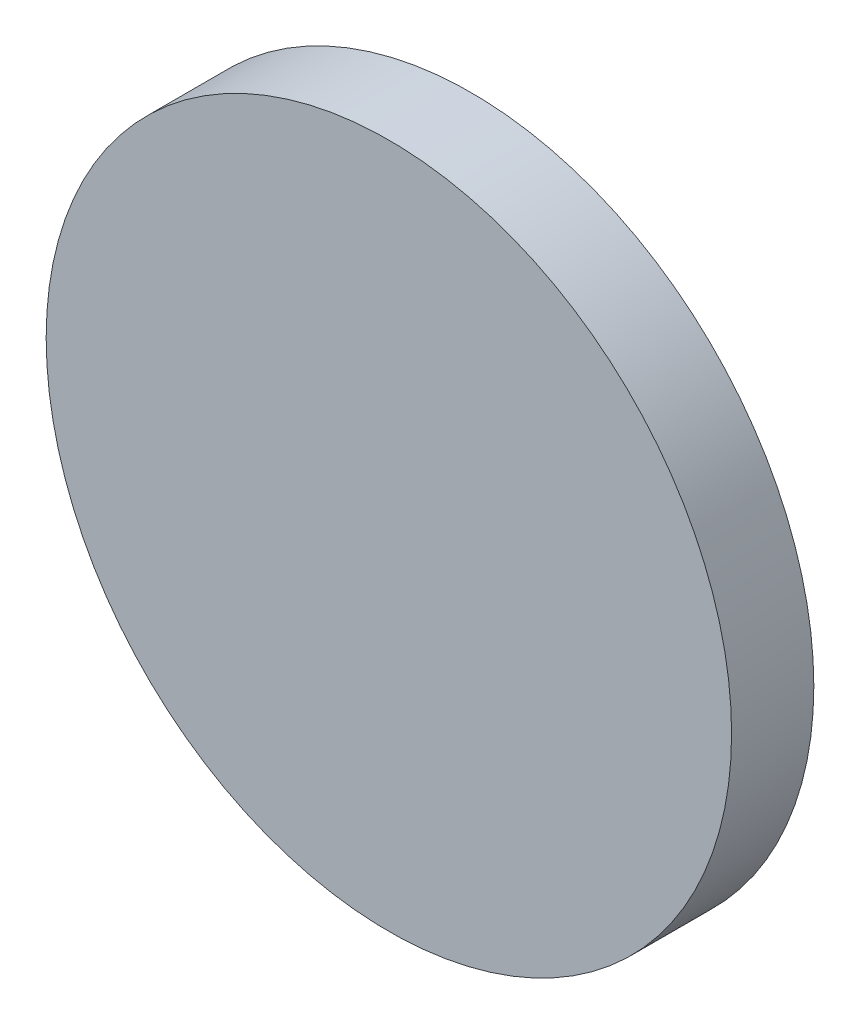
from build123d import *

# Parameters (mm, degrees)
SKETCH_1_R      = 25
EXTRUDE_1_DEPTH = 6


with BuildPart() as part:
    # 草图1 → 凸台-拉伸1 (new body)
    with BuildSketch(Plane.XY):
        Circle(SKETCH_1_R)
    extrude(amount=EXTRUDE_1_DEPTH)


solid = part.part
